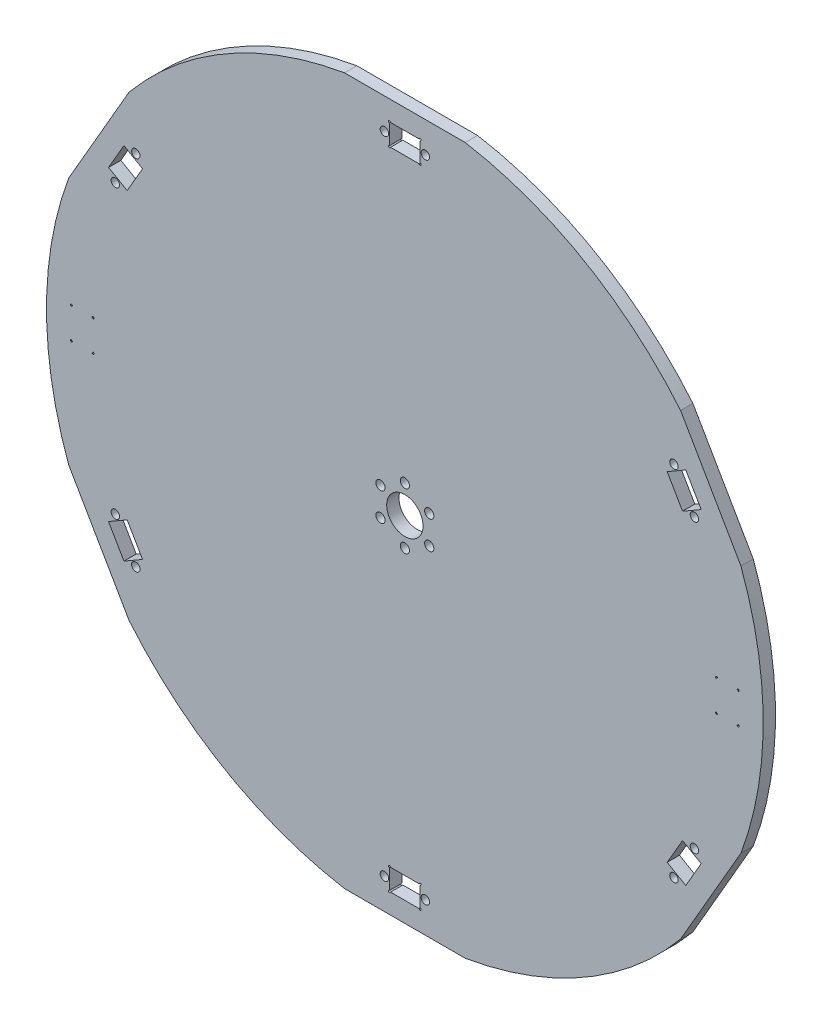
from build123d import *

# Parameters (mm, degrees)
SKETCH_1_R                       = 350
SKETCH_1_R_2                     = 17.75
EXTRUDE_1_DEPTH                  = 6
CUT_EXTRUDE_1_REACH              = 497.12
SKETCH_2_W                       = 117.898261226
SKETCH_2_H                       = 10
PATTERN_CIRCULAR_1_COUNT         = 6
CUT_EXTRUDE_2_REACH              = 493.598
SKETCH_3_W                       = 30
SKETCH_3_H                       = 21
PATTERN_CIRCULAR_2_COUNT         = 6
HOLE_WIZARD_M8_1_D               = 9
PATTERN_CIRCULAR_3_COUNT         = 6
HOLE_WIZARD_8_2_8_2_1_AT_2_COUNT = 2
HOLE_WIZARD_8_2_8_2_1_AT_2_PITCH = 40
PATTERN_CIRCULAR_5_COUNT         = 6
CUT_EXTRUDE_3_REACH              = 493.598
SKETCH_15_R                      = 1
PATTERN_CIRCULAR_6_COUNT         = 4


with BuildPart() as part:
    # 草图1 → 凸台-拉伸1 (new, symmetric)
    with BuildSketch(Plane.XY):
        Circle(SKETCH_1_R)
        Circle(SKETCH_1_R_2, mode=Mode.SUBTRACT)
    extrude(amount=EXTRUDE_1_DEPTH, both=True)

    # 草图2 → 切除-拉伸1 (cut, up to next)
    with BuildSketch(Plane.XY.offset(6), mode=Mode.PRIVATE) as cut_extrude_1_sk1:
        with Locations((0, -350)):
            Rectangle(SKETCH_2_W, SKETCH_2_H)
    cut_extrude_1_tool1 = extrude(cut_extrude_1_sk1.sketch, amount=-CUT_EXTRUDE_1_REACH, mode=Mode.PRIVATE) & part.part
    cut_extrude_1 = cut_extrude_1_tool1.solids().sort_by_distance((0, -350, 6))[0]
    add(cut_extrude_1, mode=Mode.SUBTRACT)

    # 阵列(圆周)1: 切除-拉伸1 ×6 about axis
    pattern_circular_1_axis = Axis((0, 0, 0), (0, 0, 1))
    for i in range(1, PATTERN_CIRCULAR_1_COUNT):
        add(cut_extrude_1.rotate(pattern_circular_1_axis, i * 360 / PATTERN_CIRCULAR_1_COUNT), mode=Mode.SUBTRACT)

    # 草图3 → 切除-拉伸2 (cut, up to next)
    with BuildSketch(Plane.XY.offset(6), mode=Mode.PRIVATE) as cut_extrude_2_sk1:
        with Locations((0, -315)):
            Rectangle(SKETCH_3_W, SKETCH_3_H)
    cut_extrude_2_tool1 = extrude(cut_extrude_2_sk1.sketch, amount=-CUT_EXTRUDE_2_REACH, mode=Mode.PRIVATE) & part.part
    cut_extrude_2 = cut_extrude_2_tool1.solids().sort_by_distance((0, -315, 6))[0]
    add(cut_extrude_2, mode=Mode.SUBTRACT)

    # 阵列(圆周)2: 切除-拉伸2 ×6 about axis
    pattern_circular_2_axis = Axis((0, 0, 0), (0, 0, 1))
    for i in range(1, PATTERN_CIRCULAR_2_COUNT):
        add(cut_extrude_2.rotate(pattern_circular_2_axis, i * 360 / PATTERN_CIRCULAR_2_COUNT), mode=Mode.SUBTRACT)

    # M8 间隙孔1 (through all)
    with Locations(Plane.XY.offset(6)):
        with Locations((-23.815698604, -13.75)):
            hole_wizard_m8_1 = Hole(HOLE_WIZARD_M8_1_D / 2)

    # 阵列(圆周)3: M8 间隙孔1 ×6 about axis
    pattern_circular_3_axis = Axis((0, 0, 0), (0, 0, 1))
    for i in range(1, PATTERN_CIRCULAR_3_COUNT):
        add(hole_wizard_m8_1.rotate(pattern_circular_3_axis, i * 360 / PATTERN_CIRCULAR_3_COUNT), mode=Mode.SUBTRACT)

    # 草图14 → Ø8.2 (8.2) 直径孔1 (revolve, cut)
    with BuildSketch(Plane(origin=(-20, -315, 6), x_dir=(0, -1, 0), z_dir=(1, 0, 0))):
        Polygon((0, 0), (0, 10.463528538), (4.1, 8), (4.1, 0), align=None)
    hole_wizard_8_2_8_2_1 = revolve(axis=Axis((-20, -315, 12.35), (0, 0, -1)), mode=Mode.SUBTRACT)

    # Ø8.2 (8.2) 直径孔1 at 2: Ø8.2 (8.2) 直径孔1 ×2
    with Locations(*[(i * HOLE_WIZARD_8_2_8_2_1_AT_2_PITCH, 0, 0) for i in range(1, HOLE_WIZARD_8_2_8_2_1_AT_2_COUNT)]):
        add(hole_wizard_8_2_8_2_1, mode=Mode.SUBTRACT)

    # 阵列(圆周)5: Ø8.2 (8.2) 直径孔1 ×6 about axis
    pattern_circular_5_axis = Axis((0, 0, 0), (0, 0, 1))
    for i in range(1, PATTERN_CIRCULAR_5_COUNT):
        add(hole_wizard_8_2_8_2_1.rotate(pattern_circular_5_axis, i * 360 / PATTERN_CIRCULAR_5_COUNT), mode=Mode.SUBTRACT)

    # 阵列(圆周)5 copy 1 sketch → 阵列(圆周)5 copy 1 (revolve, cut)
    with BuildSketch(Plane(origin=(282.798002192, -140.179491924, 6), x_dir=(0.8660254037844386, -0.5000000000000001, 0), z_dir=(0.5000000000000001, 0.8660254037844386, 0))):
        Polygon((0, 0), (0, 10.463528538), (4.1, 8), (4.1, 0), align=None)
    revolve(axis=Axis((282.798002192, -140.179491924, 12.35), (0, 0, -1)), mode=Mode.SUBTRACT)

    # 阵列(圆周)5 copy 2 sketch → 阵列(圆周)5 copy 2 (revolve, cut)
    with BuildSketch(Plane(origin=(262.798002192, 174.820508076, 6), x_dir=(0.8660254037844387, 0.4999999999999998, 0), z_dir=(-0.4999999999999998, 0.8660254037844387, 0))):
        Polygon((0, 0), (0, 10.463528538), (4.1, 8), (4.1, 0), align=None)
    revolve(axis=Axis((262.798002192, 174.820508076, 12.35), (0, 0, -1)), mode=Mode.SUBTRACT)

    # 阵列(圆周)5 copy 3 sketch → 阵列(圆周)5 copy 3 (revolve, cut)
    with BuildSketch(Plane(origin=(-20, 315, 6), x_dir=(0, 1, 0), z_dir=(-1, 0, 0))):
        Polygon((0, 0), (0, 10.463528538), (4.1, 8), (4.1, 0), align=None)
    revolve(axis=Axis((-20, 315, 12.35), (0, 0, -1)), mode=Mode.SUBTRACT)

    # 阵列(圆周)5 copy 4 sketch → 阵列(圆周)5 copy 4 (revolve, cut)
    with BuildSketch(Plane(origin=(-282.798002192, 140.179491924, 6), x_dir=(-0.8660254037844384, 0.5000000000000004, 0), z_dir=(-0.5000000000000004, -0.8660254037844384, 0))):
        Polygon((0, 0), (0, 10.463528538), (4.1, 8), (4.1, 0), align=None)
    revolve(axis=Axis((-282.798002192, 140.179491924, 12.35), (0, 0, -1)), mode=Mode.SUBTRACT)

    # 阵列(圆周)5 copy 5 sketch → 阵列(圆周)5 copy 5 (revolve, cut)
    with BuildSketch(Plane(origin=(-262.798002192, -174.820508076, 6), x_dir=(-0.8660254037844386, -0.5000000000000001, 0), z_dir=(0.5000000000000001, -0.8660254037844386, 0))):
        Polygon((0, 0), (0, 10.463528538), (4.1, 8), (4.1, 0), align=None)
    revolve(axis=Axis((-262.798002192, -174.820508076, 12.35), (0, 0, -1)), mode=Mode.SUBTRACT)

    # 草图15 → 切除-拉伸3 (cut, up to next)
    with BuildSketch(Plane.XY.offset(6), mode=Mode.PRIVATE) as cut_extrude_3_sk1:
        with Locations((-15, -325.5)):
            Circle(SKETCH_15_R)
    cut_extrude_3_tool1 = extrude(cut_extrude_3_sk1.sketch, amount=-CUT_EXTRUDE_3_REACH, mode=Mode.PRIVATE) & part.part
    # 草图15 → 切除-拉伸3 (cut, up to next)
    with BuildSketch(Plane.XY.offset(6), mode=Mode.PRIVATE) as cut_extrude_3_sk2:
        with Locations((15, -325.5)):
            Circle(SKETCH_15_R)
    cut_extrude_3_tool2 = extrude(cut_extrude_3_sk2.sketch, amount=-CUT_EXTRUDE_3_REACH, mode=Mode.PRIVATE) & part.part
    # 草图15 → 切除-拉伸3 (cut, up to next)
    with BuildSketch(Plane.XY.offset(6), mode=Mode.PRIVATE) as cut_extrude_3_sk3:
        with Locations((-15, -304.5)):
            Circle(SKETCH_15_R)
    cut_extrude_3_tool3 = extrude(cut_extrude_3_sk3.sketch, amount=-CUT_EXTRUDE_3_REACH, mode=Mode.PRIVATE) & part.part
    # 草图15 → 切除-拉伸3 (cut, up to next)
    with BuildSketch(Plane.XY.offset(6), mode=Mode.PRIVATE) as cut_extrude_3_sk4:
        with Locations((15, -304.5)):
            Circle(SKETCH_15_R)
    cut_extrude_3_tool4 = extrude(cut_extrude_3_sk4.sketch, amount=-CUT_EXTRUDE_3_REACH, mode=Mode.PRIVATE) & part.part
    cut_extrude_3_1 = cut_extrude_3_tool1.solids().sort_by_distance((-15, -325.5, 6))[0]
    add(cut_extrude_3_1, mode=Mode.SUBTRACT)
    cut_extrude_3_2 = cut_extrude_3_tool2.solids().sort_by_distance((15, -325.5, 6))[0]
    add(cut_extrude_3_2, mode=Mode.SUBTRACT)
    cut_extrude_3_3 = cut_extrude_3_tool3.solids().sort_by_distance((-15, -304.5, 6))[0]
    add(cut_extrude_3_3, mode=Mode.SUBTRACT)
    cut_extrude_3_4 = cut_extrude_3_tool4.solids().sort_by_distance((15, -304.5, 6))[0]
    add(cut_extrude_3_4, mode=Mode.SUBTRACT)
    cut_extrude_3 = cut_extrude_3_1 + cut_extrude_3_2 + cut_extrude_3_3 + cut_extrude_3_4  # 切除-拉伸3 as one shape, for the pattern or mirror that repeats it

    # 阵列(圆周)6: 切除-拉伸3 ×4 about axis
    pattern_circular_6_axis = Axis((0, 0, 0), (0, 0, 1))
    for i in range(1, PATTERN_CIRCULAR_6_COUNT):
        add(cut_extrude_3.rotate(pattern_circular_6_axis, i * 360 / PATTERN_CIRCULAR_6_COUNT), mode=Mode.SUBTRACT)


solid = part.part
